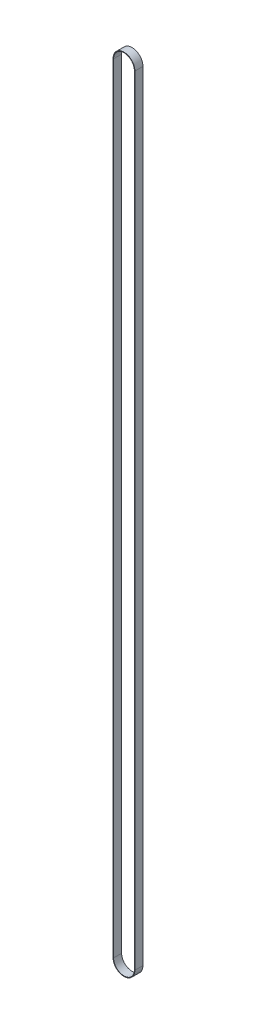
SolidWorks part; units mm, degrees
ref_plane "前视基准面" through (0, 0, 0) normal (0, 0, 1) x (1, 0, 0)
ref_plane "上视基准面" through (0, 0, 0) normal (0, 1, 0) x (1, 0, 0)
ref_plane "右视基准面" through (0, 0, 0) normal (1, 0, 0) x (0, 0, -1)
sketch "草图2" plane through (0, 0, 0) normal (0, 0, 1) x (1, 0, 0)
  line L0 (0, 0) -> (1, 0) construction
  line L1 (0, 0) -> (0, 1) construction
  line L2 (-19.415, 0) -> (-19.415, 1455)
  line L3 (19.415, 1455) -> (19.415, 0)
  arc A0 (19.415, 0) -> (-19.415, 0) centre (0, 0) cw
  arc A1 (-19.415, 1455) -> (19.415, 1455) centre (0, 1455) cw
extrude "拉伸-薄壁1" add sketch "草图2" along normal mid plane 15 thin thin type one direction wall 1
